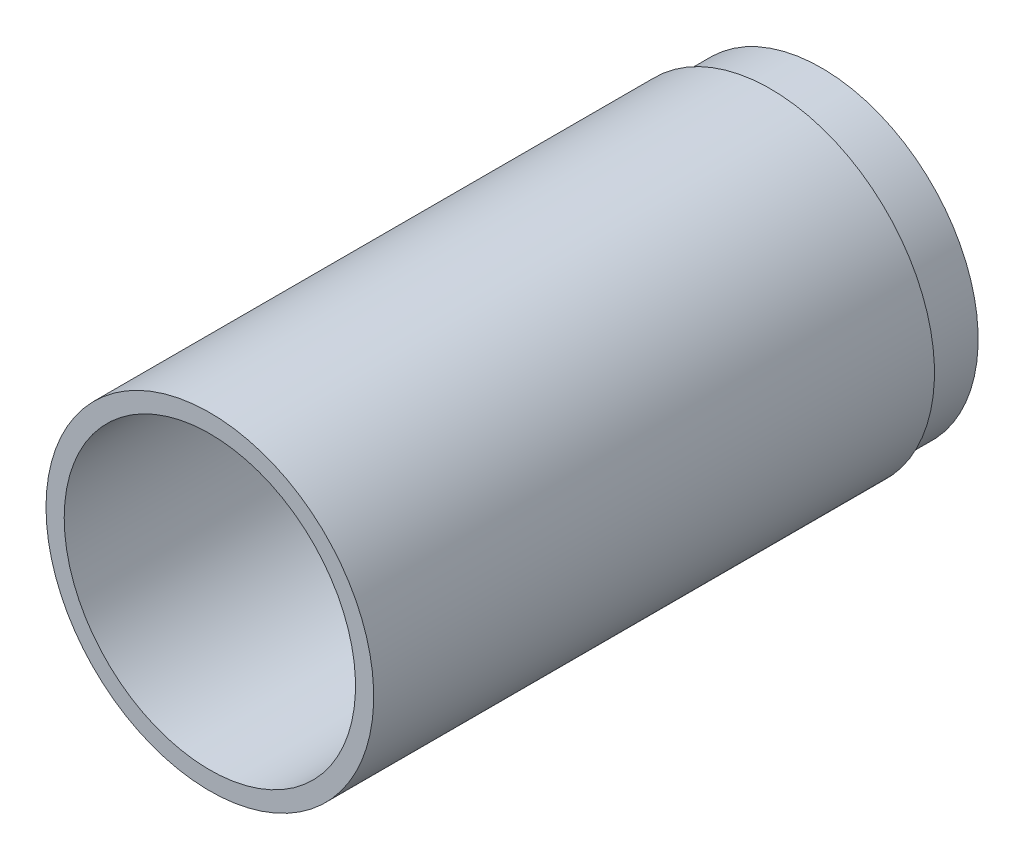
from build123d import *

# Parameters (mm, degrees)
SKETCH1_R           = 22.5
SKETCH1_R_2         = 20
BOSS_EXTRUDE1_DEPTH = 84
SKETCH2_R           = 22.5
SKETCH2_R_2         = 21.5
CUT_EXTRUDE1_DEPTH  = 7


with BuildPart() as part:
    # Sketch1 → Boss-Extrude1 (new body)
    with BuildSketch(Plane.XY):
        with Locations(Location((0, 0, 0), (0, 0, 180))):
            Circle(SKETCH1_R)
        with Locations(Location((0, 0, 0), (0, 0, 180))):
            Circle(SKETCH1_R_2, mode=Mode.SUBTRACT)
    extrude(amount=BOSS_EXTRUDE1_DEPTH)

    # Sketch2 → Cut-Extrude1 (cut)
    with BuildSketch(Plane(origin=(0, 0, 0), x_dir=(-1, 0, 0), z_dir=(0, 0, -1))):
        Circle(SKETCH2_R)
        Circle(SKETCH2_R_2, mode=Mode.SUBTRACT)
    extrude(amount=-CUT_EXTRUDE1_DEPTH, mode=Mode.SUBTRACT)


solid = part.part
